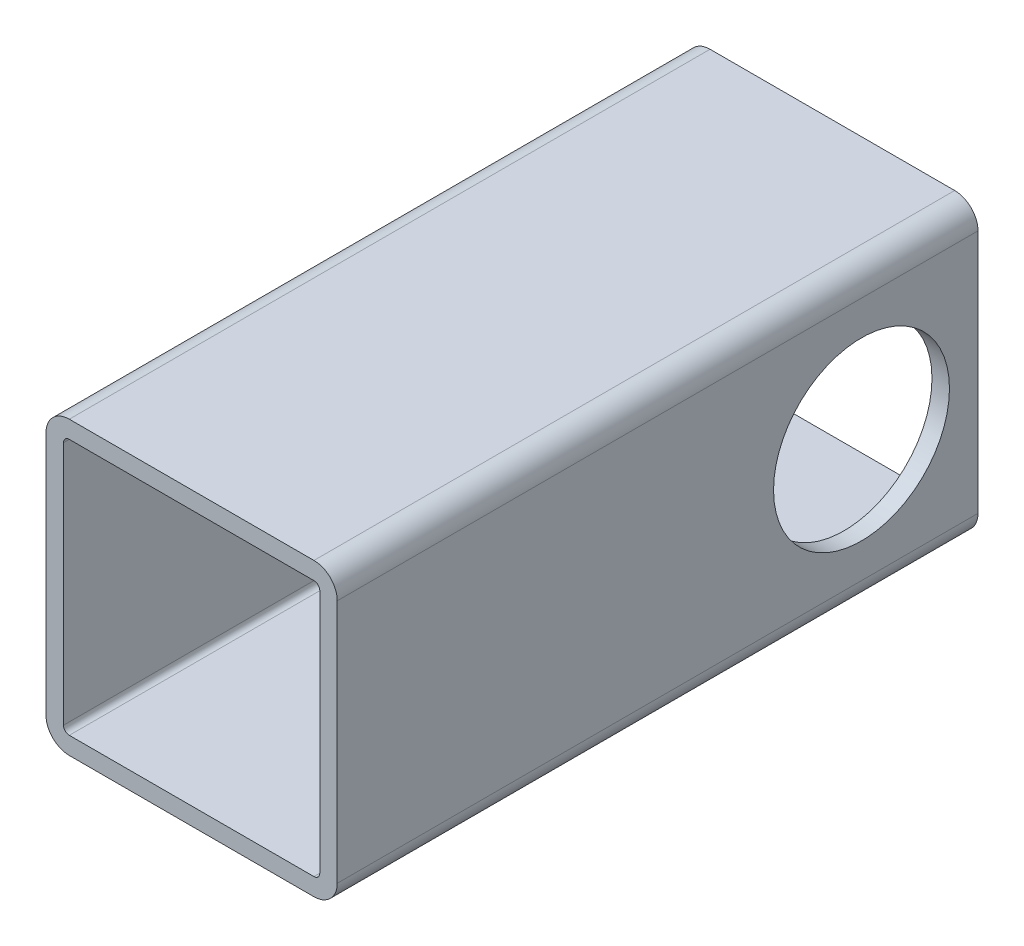
SolidWorks part; units mm, degrees
material "AISI 1045 钢，冷拔"
ref_plane "Front Plane" through (0, 0, 0) normal (0, 0, 1) x (1, 0, 0)
ref_plane "Top Plane" through (0, 0, 0) normal (0, 1, 0) x (1, 0, 0)
ref_plane "Right Plane" through (0, 0, 0) normal (1, 0, 0) x (0, 0, -1)
sketch "Sketch1" plane through (0, 0, 0) normal (0, 0, 1) x (1, 0, 0)
  line L1 (-21, -25) -> (21, -25)
  line L2 (-25, -21) -> (-25, 21)
  line L3 (-21, 25) -> (21, 25)
  line L4 (25, -21) -> (25, 21)
  line L5 (-25, -25) -> (25, 25) construction
  line L6 (-25, 25) -> (25, -25) construction
  arc A0 (-21, -25) -> (-25, -21) centre (-21, -21) cw
  arc A1 (21, -25) -> (25, -21) centre (21, -21) ccw
  arc A2 (21, 25) -> (25, 21) centre (21, 21) cw
  arc A3 (-25, 21) -> (-21, 25) centre (-21, 21) cw
  point P0 (0, 0)
  dimension "D3" = 4
  dimension "D1" = 50
  dimension "D2" = 50
extrude "Extrude-Thin1" add sketch "Sketch1" along normal blind 110 thin thin type one direction reverse wall 3
sketch "Sketch2" plane through (25, 0, 0) normal (1, 0, 0) x (0, 0, -1)
  line L0 (0, -21) -> (0, 21) construction
  line L1 (-110, 25) -> (0, 25) construction
  circle A0 centre (-20, 0) radius 15.1
  dimension "D1" = 30.2
  dimension "D2" = 20
  dimension "D3" = 25
extrude "Cut-Extrude1" cut sketch "Sketch2" against normal through all
